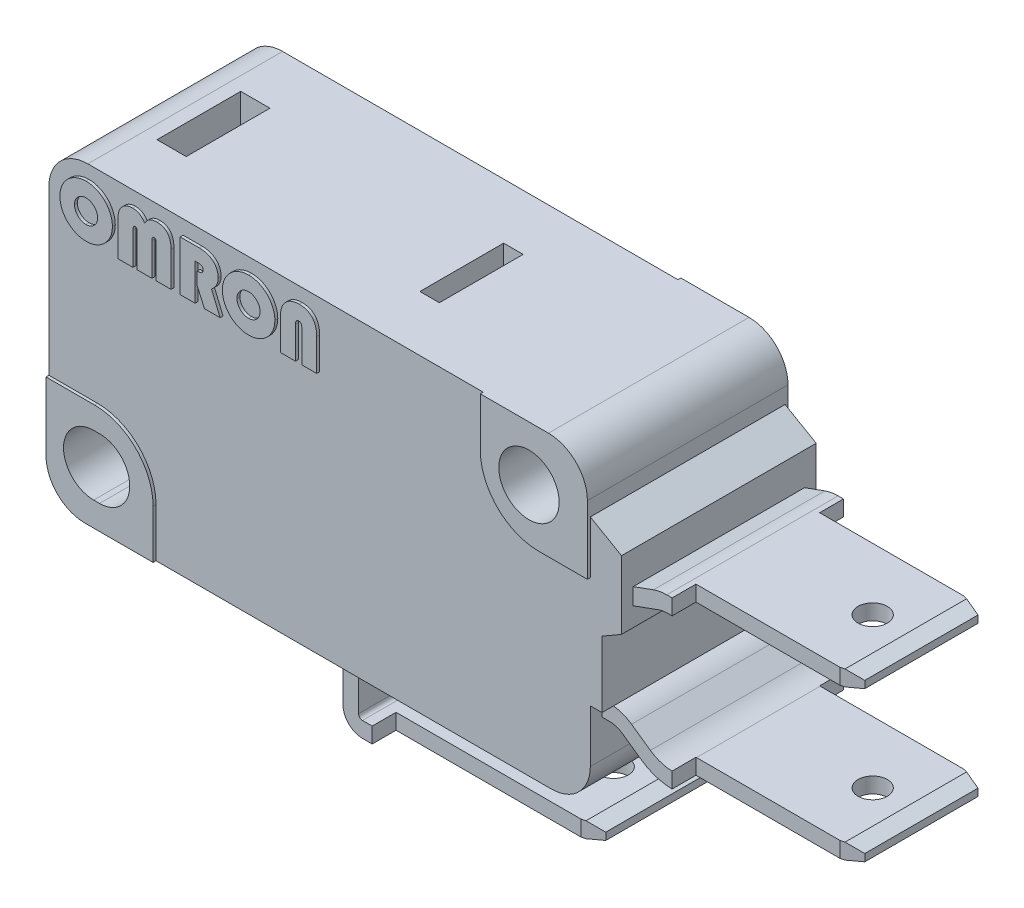
SolidWorks part; units mm, degrees
material "CA"
ref_plane "前视基准面" through (0, 0, 0) normal (0, 0, 1) x (1, 0, 0)
ref_plane "上视基准面" through (0, 0, 0) normal (0, 1, 0) x (1, 0, 0)
ref_plane "右视基准面" through (0, 0, 0) normal (1, 0, 0) x (0, 0, -1)
sketch "草图1" plane through (0, 0, 0) normal (0, 0, 1) x (1, 0, 0)
  line L0 (-16.5607, 0) -> (15.8247, 0) construction
  line L1 (0, 10.5498) -> (0, -11.5312) construction
  line L2 (13.9, -3.25) -> (14.5, -3.25)
  line L3 (-11.9, 7.95) -> (11.9, 7.95)
  line L4 (-13.9, 5.95) -> (-13.9, -5.95)
  line L5 (-11.9, -7.95) -> (11.9, -7.95)
  line L6 (13.9, 5.95) -> (13.9, 5.15)
  line L7 (14.5, -3.25) -> (14.5, 0.1489)
  line L8 (14.5, 0.1489) -> (15.5, 0.7262)
  line L9 (15.5, 0.7262) -> (15.5, 4.2262)
  line L10 (15.5, 4.2262) -> (13.9, 5.15)
  line L11 (13.9, -3.25) -> (13.9, -5.95)
  arc A0 (11.9, 7.95) -> (13.9, 5.95) centre (11.9, 5.95) cw
  arc A1 (11.9, -7.95) -> (13.9, -5.95) centre (11.9, -5.95) ccw
  arc A2 (-13.9, -5.95) -> (-11.9, -7.95) centre (-11.9, -5.95) ccw
  arc A3 (-11.9, 7.95) -> (-13.9, 5.95) centre (-11.9, 5.95) ccw
  dimension "D10" = 2
  dimension "D1" = 27.8
  dimension "D2" = 15.9
  dimension "D3" = 1.6
  dimension "D4" = 0.6
  dimension "D5" = 2.8
  dimension "D6" = 120
  dimension "D7" = 120
  dimension "D8" = 3.5
  dimension "D9" = 8.4
extrude "凸台-拉伸1" add sketch "草图1" along normal mid plane 10
sketch "草图2" plane through (0, 0, 5) normal (0, 0, 1) x (1, 0, 0)
  line L0 (-13.9, -2.45) -> (-11.4, -2.45)
  line L1 (-13.9, 5.95) -> (-13.9, -5.95) construction
  line L2 (-8.4, -5.45) -> (-8.4, -7.95)
  line L3 (-11.9, -7.95) -> (11.9, -7.95) construction
  line L4 (8.4, 7.95) -> (8.4, 5.45)
  line L5 (11.9, 7.95) -> (-11.9, 7.95) construction
  line L6 (11.4, 2.45) -> (13.9, 2.45)
  line L7 (13.9, 2.45) -> (13.9, 5.15)
  line L18 (13.9, -5.95) -> (13.9, -3.25)
  line L19 (13.9, -3.25) -> (14.5, -3.25)
  line L20 (14.5, -3.25) -> (14.5, 0.1489)
  line L21 (14.5, 0.1489) -> (15.5, 0.7262)
  line L22 (15.5, 0.7262) -> (15.5, 4.2262)
  line L23 (15.5, 4.2262) -> (13.9, 5.15)
  line L24 (13.9, 5.15) -> (13.9, 5.95)
  line L25 (11.9, 7.95) -> (-11.9, 7.95)
  line L26 (-13.9, 5.95) -> (-13.9, -5.95)
  line L27 (-11.9, -7.95) -> (11.9, -7.95)
  line L34 (13.9, 5.15) -> (13.9, 5.95)
  line L35 (11.9, 7.95) -> (8.4, 7.95)
  line L36 (-13.9, -2.45) -> (-13.9, -5.95)
  line L37 (-11.9, -7.95) -> (-8.4, -7.95)
  arc A0 (8.4, 5.45) -> (11.4, 2.45) centre (11.4, 5.45) ccw
  arc A1 (-11.4, -2.45) -> (-8.4, -5.45) centre (-11.4, -5.45) cw
  arc A4 (13.9, 5.95) -> (11.9, 7.95) centre (11.9, 5.95) ccw
  arc A5 (-11.9, 7.95) -> (-13.9, 5.95) centre (-11.9, 5.95) ccw
  arc A6 (-13.9, -5.95) -> (-11.9, -7.95) centre (-11.9, -5.95) ccw
  arc A7 (11.9, -7.95) -> (13.9, -5.95) centre (11.9, -5.95) ccw
  arc A8 (13.9, 5.95) -> (11.9, 7.95) centre (11.9, 5.95) ccw
  arc A10 (-13.9, -5.95) -> (-11.9, -7.95) centre (-11.9, -5.95) ccw
  dimension "D6" = 3
  dimension "D2" = 5.5
  dimension "D3" = 5.5
  dimension "D4" = 5.5
  dimension "D5" = 5.5
  dimension "D1" = 0
extrude "凸台-拉伸2" add sketch "草图2" along normal blind 0.15
mirror "镜向1" about plane through (0, 0, 0) normal (0, 0, 1) of "凸台-拉伸2"
sketch "草图3" plane through (0, 0, 5.15) normal (0, 0, 1) x (1, 0, 0)
  line L0 (11.9, 7.95) -> (8.4, 7.95) construction
  line L1 (13.9, 2.45) -> (13.9, 5.95) construction
  line L2 (-11.45, -5.15) -> (-11.15, -5.15) construction
  line L3 (-11.45, -3.6) -> (-11.15, -3.6)
  line L4 (-11.45, -6.7) -> (-11.15, -6.7)
  circle A0 centre (10.9, 5.15) radius 1.55
  arc A1 (-11.45, -3.6) -> (-11.45, -6.7) centre (-11.45, -5.15) ccw
  arc A2 (-11.15, -6.7) -> (-11.15, -3.6) centre (-11.15, -5.15) ccw
  point P8 (-11.3, -5.15)
  dimension "D1" = 3.1
  dimension "D2" = 2.8
  dimension "D3" = 3
  dimension "D5" = 3.4
  dimension "D7" = 10.3
  dimension "D4" = 3.1
  dimension "D6" = 22.2
extrude "切除-拉伸1" cut sketch "草图3" against normal through all
sketch "草图5" plane through (0, 0, 0) normal (0, 0, 1) x (1, 0, 0)
  line L0 (8.4, 7.95) -> (-11.9, 7.95) construction
  line L1 (-11.2, 7.95) -> (-9.7, 7.95)
  line L2 (-11.2, 7.95) -> (-11.2, 3.45)
  line L3 (-13.9, 5.95) -> (-13.9, -2.45) construction
  line L4 (-9.7, 7.95) -> (-9.7, 3.45)
  line L5 (11.9, 7.95) -> (8.4, 7.95) construction
  line L6 (2.3, 7.95) -> (3.3, 7.95)
  line L7 (2.3, 7.95) -> (2.3, 6.05)
  line L8 (2.8, 6.05) -> (2.8, 9.2487) construction
  line L9 (3.3, 7.95) -> (3.3, 6.05)
  arc A0 (-11.2, 3.45) -> (-9.7, 3.45) centre (-10.45, 3.45) ccw
  arc A1 (2.3, 6.05) -> (3.3, 6.05) centre (2.8, 6.05) ccw
  circle A3 centre (10.9, 5.15) radius 1.55 construction
  dimension "D6" = 1.9
  dimension "D1" = 4.5
  dimension "D2" = 2.7
  dimension "D3" = 1.5
  dimension "D4" = 8.1
  dimension "D5" = 1
extrude "切除-拉伸2" cut sketch "草图5" against normal mid plane 4.3
sketch "草图8" plane through (0, 0, 0) normal (0, 0, 1) x (1, 0, 0)
  circle A0 centre (2.8, 6.05) radius 0.5
  dimension "D1" = 1
extrude "切除-拉伸3" cut sketch "草图8" against normal mid plane 6
sketch "草图9" plane through (0, 0, 0) normal (0, 0, 1) x (1, 0, 0)
  line L0 (0.6, -7.95) -> (0.6, -10.15)
  line L1 (-8.4, -7.95) -> (11.9, -7.95) construction
  line L2 (1.6, -11.15) -> (12.6, -11.15)
  line L3 (13.9, -3.25) -> (14.2694, -3.25)
  line L4 (15.4166, -3.6117) -> (16.3829, -4.2883)
  line L5 (17.53, -4.65) -> (25.9, -4.65)
  line L6 (15.5, 2.55) -> (16.5424, 2.9294)
  line L7 (15.5, 0.7262) -> (15.5, 4.2262) construction
  line L8 (17.2264, 3.05) -> (25.9, 3.05)
  line L9 (-13.9, -2.45) -> (-13.9, -5.95) construction
  line L10 (11.9, 7.95) -> (8.4, 7.95) construction
  line L11 (1.4, -7.95) -> (1.4, -10.15)
  line L12 (1.6, -10.35) -> (12.6, -10.35)
  line L13 (12.6, -10.35) -> (12.6, -11.15)
  line L14 (0.6, -7.95) -> (1.4, -7.95)
  line L15 (15.5, 1.6987) -> (16.816, 2.1776)
  line L16 (17.2264, 2.25) -> (25.9, 2.25)
  line L17 (13.9, -4.05) -> (14.2694, -4.05)
  line L18 (14.9577, -4.267) -> (15.924, -4.9436)
  line L19 (17.53, -5.45) -> (25.9, -5.45)
  line L20 (15.5, 2.55) -> (15.5, 1.6987)
  line L21 (13.9, -3.25) -> (13.9, -4.05)
  line L22 (25.9, 3.05) -> (25.9, 2.25)
  line L23 (25.9, -4.65) -> (25.9, -5.45)
  line L24 (15.7736, 1.7982) -> (16.816, 2.1776) construction
  arc A0 (0.6, -10.15) -> (1.6, -11.15) centre (1.6, -10.15) ccw
  arc A1 (1.4, -10.15) -> (1.6, -10.35) centre (1.6, -10.15) ccw
  arc A2 (14.2694, -3.25) -> (15.4166, -3.6117) centre (14.2694, -5.25) cw
  arc A3 (16.3829, -4.2883) -> (17.53, -4.65) centre (17.53, -2.65) ccw
  arc A4 (16.5424, 2.9294) -> (17.2264, 3.05) centre (17.2264, 1.05) cw
  arc A5 (16.816, 2.1776) -> (17.2264, 2.25) centre (17.2264, 1.05) cw
  arc A6 (14.2694, -4.05) -> (14.9577, -4.267) centre (14.2694, -5.25) cw
  arc A7 (15.924, -4.9436) -> (17.53, -5.45) centre (17.53, -2.65) ccw
  point P28 (14.9, -3.25)
  dimension "D4" = 1
  dimension "D12" = 2
  dimension "D1" = 14.5
  dimension "D2" = 19.1
  dimension "D3" = 12
  dimension "D6" = 39.8
  dimension "D7" = 1
  dimension "D8" = 145
  dimension "D9" = 7.7
  dimension "D10" = 0.5
  dimension "D11" = 70
  dimension "D14" = 4.9
  dimension "D5" = 0.8
  dimension "D13" = 0.8
extrude "凸台-拉伸3" add sketch "草图9" along normal mid plane 8.8
sketch "草图10" plane through (0, 3.05, 0) normal (0, 1, 0) x (1, 0, 0)
  line L0 (-14.41, 0) -> (27.1507, 0) construction
  line L1 (17.5, 4.4) -> (17.5, 3.175)
  line L2 (25.9, 4.4) -> (17.2264, 4.4) construction
  line L3 (17.5, 3.175) -> (25.9, 3.175)
  line L4 (25.9, -4.4) -> (25.9, 4.4) construction
  line L5 (17.5, -3.175) -> (25.9, -3.175)
  line L6 (17.5, -4.4) -> (17.5, -3.175)
  line L7 (17.5, 4.4) -> (25.9, 4.4)
  line L8 (25.9, 4.4) -> (25.9, 3.175)
  line L9 (17.5, -4.4) -> (25.9, -4.4)
  line L10 (25.9, -4.4) -> (25.9, -3.175)
  line L11 (15.5, -5) -> (15.5, 5) construction
  circle A0 centre (23.4, 0) radius 0.75
  dimension "D3" = 1.5
  dimension "D4" = 2.5
  dimension "D1" = 6.35
  dimension "D2" = 2
extrude "切除-拉伸4" cut sketch "草图10" against normal through all
sketch "草图11" plane through (0, -11.15, 0) normal (0, -1, 0) x (1, 0, 0)
  line L0 (2.1, 4.4) -> (2.1, 3.175)
  line L1 (1.6, 4.4) -> (12.6, 4.4) construction
  line L2 (2.1, 3.175) -> (12.6, 3.175)
  line L3 (12.6, 4.4) -> (12.6, -4.4) construction
  line L4 (2.1, 4.4) -> (12.6, 4.4)
  line L5 (12.6, 4.4) -> (12.6, 3.175)
  line L6 (-7.4248, 0) -> (15.3359, 0) construction
  line L7 (12.6, -4.4) -> (12.6, -3.175)
  line L8 (2.1, -4.4) -> (12.6, -4.4)
  line L9 (2.1, -3.175) -> (12.6, -3.175)
  line L10 (2.1, -4.4) -> (2.1, -3.175)
  line L11 (0.6, 4.4) -> (0.6, -4.4) construction
  circle A0 centre (10.1, 0) radius 0.75
  dimension "D1" = 2.5
  dimension "D2" = 1.5
  dimension "D3" = 6.35
  dimension "D4" = 1.5
extrude "切除-拉伸5" cut sketch "草图11" against normal blind 1
chamfer "倒角1" distance 0.8 angle 15 3 edges at (25.9, -4.65, 0) (25.9, 3.05, 0) (12.6, -10.35, 0)
chamfer "倒角2" distance 0.8 angle 15 3 edges at (25.9, -5.45, 0) (25.9, 2.25, 0) (12.6, -11.15, 0)
chamfer "倒角3" distance 1 angle 15 3 edges at (25.9, -5.05, -3.175) (25.9, 2.65, -3.175) (12.6, -10.75, -3.175)
chamfer "倒角4" distance 1 angle 15 3 edges at (25.9, -5.05, 3.175) (25.9, 2.65, 3.175) (12.6, -10.75, 3.175)
sketch "草图12" plane through (0, 0, 5) normal (0, 0, 1) x (1, 0, 0)
  text T0 "OMRON" font "华文琥珀" height in points 10
extrude "凸台-拉伸6" add sketch "草图12" along normal blind 0.15
